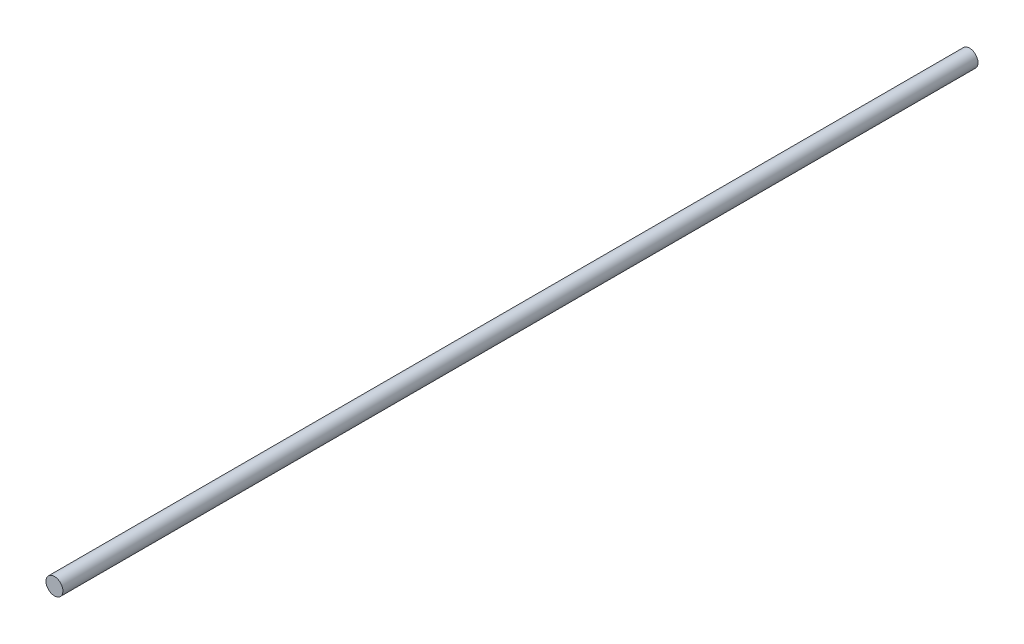
SolidWorks part; units mm, degrees
ref_plane "前视基准面" through (0, 0, 0) normal (0, 0, 1) x (1, 0, 0)
ref_plane "上视基准面" through (0, 0, 0) normal (0, 1, 0) x (1, 0, 0)
ref_plane "右视基准面" through (0, 0, 0) normal (1, 0, 0) x (0, 0, -1)
sketch "草图1" plane through (0, 0, 0) normal (0, 0, 1) x (1, 0, 0)
  circle A0 centre (0, 0) radius 12.5
  dimension "D1" = 25
extrude "凸台-拉伸1" add sketch "草图1" along normal blind 1352
